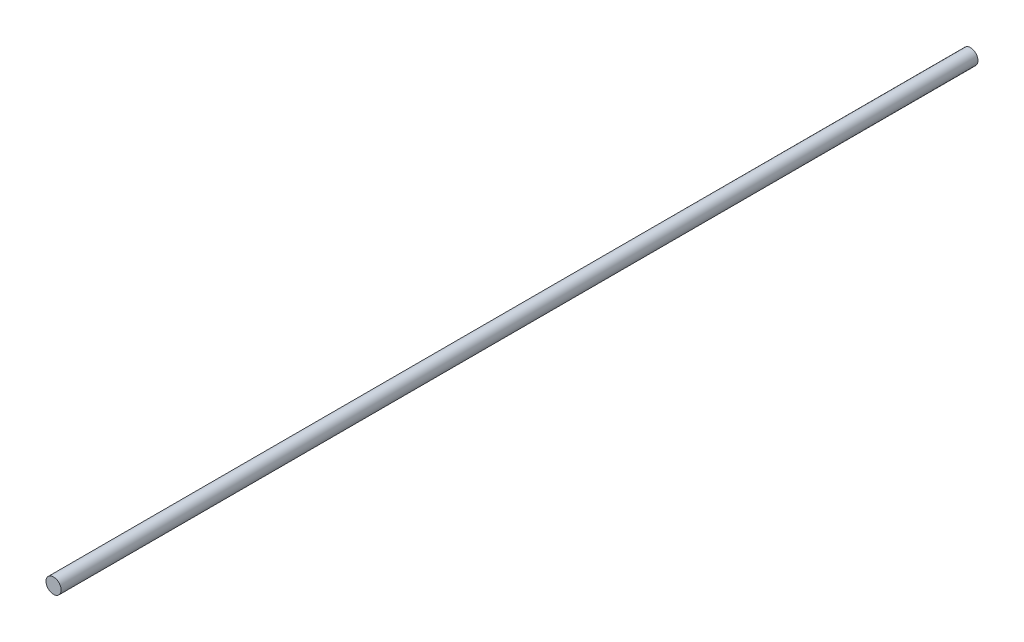
SolidWorks part; units mm, degrees
material "SWM-B"
ref_plane "Front Plane" through (0, 0, 0) normal (0, 0, 1) x (1, 0, 0)
ref_plane "Top Plane" through (0, 0, 0) normal (0, 1, 0) x (1, 0, 0)
ref_plane "Right Plane" through (0, 0, 0) normal (1, 0, 0) x (0, 0, -1)
sketch "Sketch1" plane through (0, 0, 0) normal (0, 0, 1) x (1, 0, 0)
  circle A0 centre (0, 0) radius 2
  dimension "D1" = 4
extrude "Boss-Extrude1" add sketch "Sketch1" along normal blind 242.5
